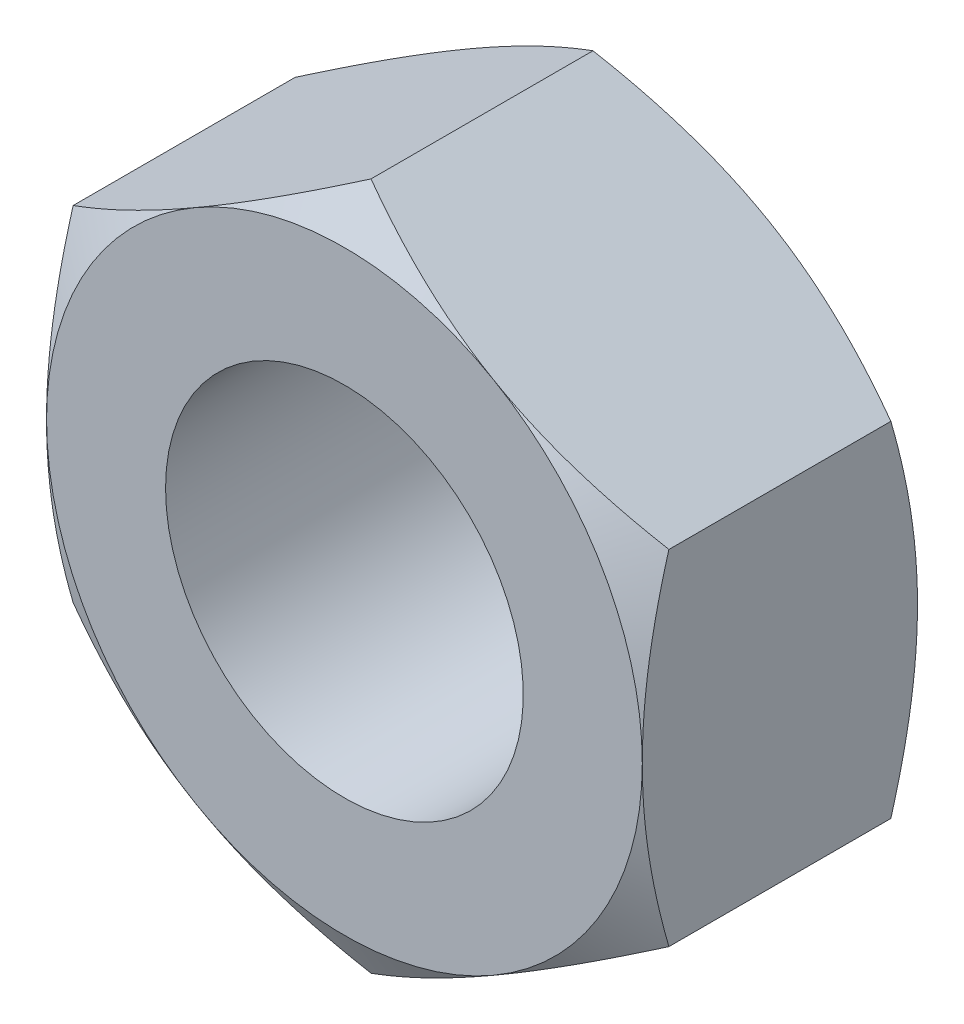
from build123d import *

# Parameters (mm, degrees)
BOSS_EXTRUDE1_DEPTH     = 5
SKETCH2_OUTSIDE_W       = 65.202
SKETCH2_OUTSIDE_H       = 68.552
SKETCH2_OUTSIDE_R       = 10.825317547
CUT_EXTRUDE1_DEPTH      = 10
CUT_EXTRUDE1_DRAFT      = -60
MIRROR1_COPY_1_SKETCH_W = 65.202
MIRROR1_COPY_1_SKETCH_H = 68.552
MIRROR1_COPY_1_SKETCH_R = 10.825317547
MIRROR1_COPY_1_DEPTH    = 10
MIRROR1_COPY_1_DRAFT    = -60
SKETCH3_R               = 6.5
CUT_EXTRUDE2_DEPTH      = 10


with BuildPart() as part:
    # Sketch1 → Boss-Extrude1 (new, symmetric)
    with BuildSketch(Plane.XY):
        Polygon((0, 12.5), (-10.825317547, 6.25), (-10.825317547, -6.25), (0, -12.5), (10.825317547, -6.25), (10.825317547, 6.25), align=None)
    extrude(amount=BOSS_EXTRUDE1_DEPTH, both=True)


with BuildPart() as cut_extrude1_tool:
    # Sketch2 outside → Cut-Extrude1 (with draft: the straight prism first)
    with BuildSketch(Plane.XY.offset(5)):
        Rectangle(SKETCH2_OUTSIDE_W, SKETCH2_OUTSIDE_H)
        Circle(SKETCH2_OUTSIDE_R, mode=Mode.SUBTRACT)
    extrude(amount=-CUT_EXTRUDE1_DEPTH)
    # Cut-Extrude1: the draft: its side faces are tilted about the plane it starts from
    cut_extrude1_sides = [cut_extrude1_tool.faces().sort_by_distance(p)[0] for p in [
        (0, -34.276, 0),
        (32.601, 0, 0),
        (0, 34.276, 0),
        (-32.601, 0, 0),
        (-10.825317547, 0, 0),
    ]]
    draft(cut_extrude1_sides, Plane.XY.offset(5), CUT_EXTRUDE1_DRAFT)


with BuildPart() as part_1:
    add(part.part)

    # Cut-Extrude1: cut by cut_extrude1_tool
    add(cut_extrude1_tool.part, mode=Mode.SUBTRACT)


with BuildPart() as mirror1_copy_1_tool:
    # Mirror1 copy 1 sketch → Mirror1 copy 1 (with draft: the straight prism first)
    with BuildSketch(Plane(origin=(0, 0, -5), x_dir=(1, 0, 0), z_dir=(0, 0, -1))):
        Rectangle(MIRROR1_COPY_1_SKETCH_W, MIRROR1_COPY_1_SKETCH_H)
        Circle(MIRROR1_COPY_1_SKETCH_R, mode=Mode.SUBTRACT)
    extrude(amount=-MIRROR1_COPY_1_DEPTH)
    # Mirror1 copy 1: the draft: its side faces are tilted about the plane it starts from
    mirror1_copy_1_sides = [mirror1_copy_1_tool.faces().sort_by_distance(p)[0] for p in [
        (0, -34.276, 0),
        (32.601, 0, 0),
        (0, 34.276, 0),
        (-32.601, 0, 0),
        (-10.825317547, 0, 0),
    ]]
    draft(mirror1_copy_1_sides, Plane(origin=(0, 0, -5), x_dir=(1, 0, 0), z_dir=(0, 0, -1)), MIRROR1_COPY_1_DRAFT)


with BuildPart() as part_2:
    add(part_1.part)

    # Mirror1 copy 1: cut by mirror1_copy_1_tool
    add(mirror1_copy_1_tool.part, mode=Mode.SUBTRACT)

    # Sketch3 → Cut-Extrude2 (cut)
    with BuildSketch(Plane(origin=(0, 0, -5), x_dir=(-1, 0, 0), z_dir=(0, 0, -1))):
        Circle(SKETCH3_R)
    extrude(amount=-CUT_EXTRUDE2_DEPTH, mode=Mode.SUBTRACT)


solid = part_2.part
